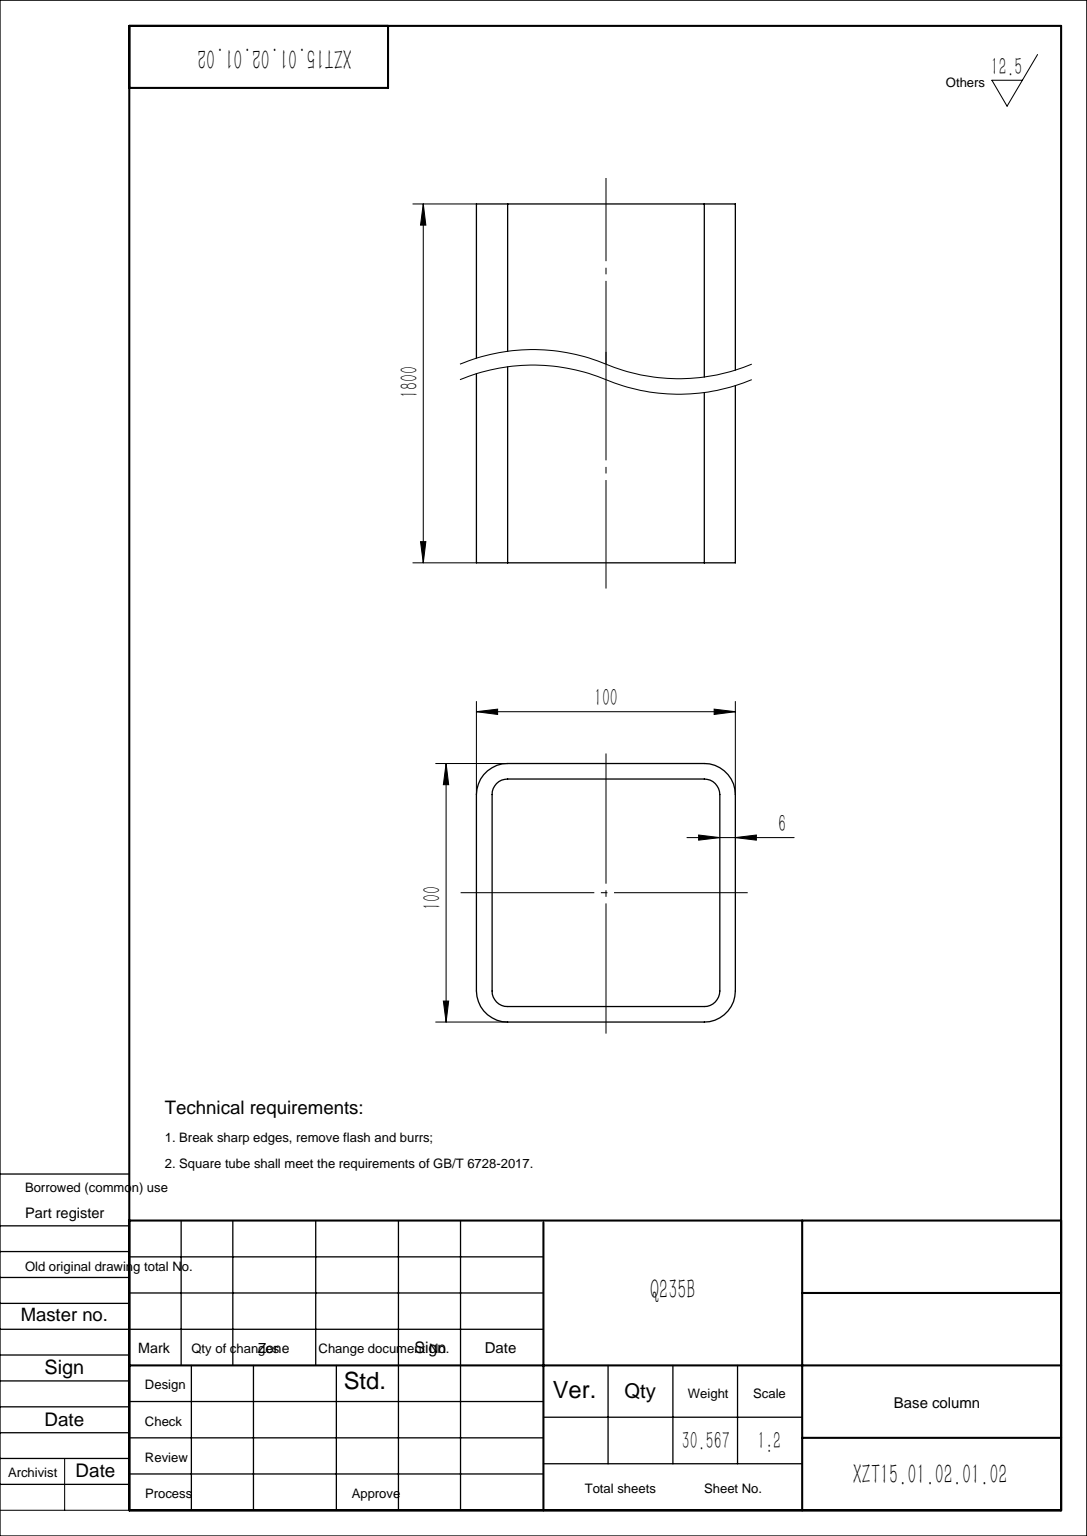
SolidWorks part; units mm, degrees
material "Q235B"
ref_plane "Front Plane" through (0, 0, 0) normal (0, 0, 1) x (1, 0, 0)
ref_plane "Top Plane" through (0, 0, 0) normal (0, 1, 0) x (1, 0, 0)
ref_plane "Right Plane" through (0, 0, 0) normal (1, 0, 0) x (0, 0, -1)
sketch "Sketch1" plane through (0, 0, 0) normal (0, 0, 1) x (1, 0, 0)
  line L0 (0, 0) -> (0, 1800)
  dimension "D1" = 1800
other "GB/T 6728-2002 square hollow section 100×100×6(1)"
ref_plane "Plane1" through (0, 0, 0) normal (0, 1, 0) x (-1, 0, 0)
sketch "Sketch11" plane through (0, 0, 0) normal (0, 1, 0) x (-1, 0, 0)
  line L0 (-38, -44) -> (38, -44)
  line L1 (-44, -38) -> (-44, 38)
  line L2 (38, 44) -> (-38, 44)
  line L3 (44, 38) -> (44, -38)
  line L4 (-38, -50) -> (38, -50)
  line L5 (-50, -38) -> (-50, 38)
  line L6 (38, 50) -> (-38, 50)
  line L7 (50, 38) -> (50, -38)
  arc A0 (50, 38) -> (38, 50) centre (38, 38) ccw
  arc A1 (38, -50) -> (50, -38) centre (38, -38) ccw
  arc A2 (-50, -38) -> (-38, -50) centre (-38, -38) ccw
  arc A3 (-38, 50) -> (-50, 38) centre (-38, 38) ccw
  arc A4 (-38, 44) -> (-44, 38) centre (-38, 38) ccw
  arc A5 (44, 38) -> (38, 44) centre (38, 38) ccw
  arc A6 (38, -44) -> (44, -38) centre (38, -38) ccw
  arc A7 (-44, -38) -> (-38, -44) centre (-38, -38) ccw
  point P0 (-50, 0)
  point P1 (50, 0)
  point P2 (0, 50)
  point P3 (0, -50)
  point P4 (0, 0)
  point P5 (-50, -50)
  point P6 (50, -50)
  point P7 (50, 50)
  point P8 (-50, 50)
  point P33 (0, 0)
  dimension "D1" = 12
  dimension "Thickness" = 6
  dimension "V_leg" = 100
